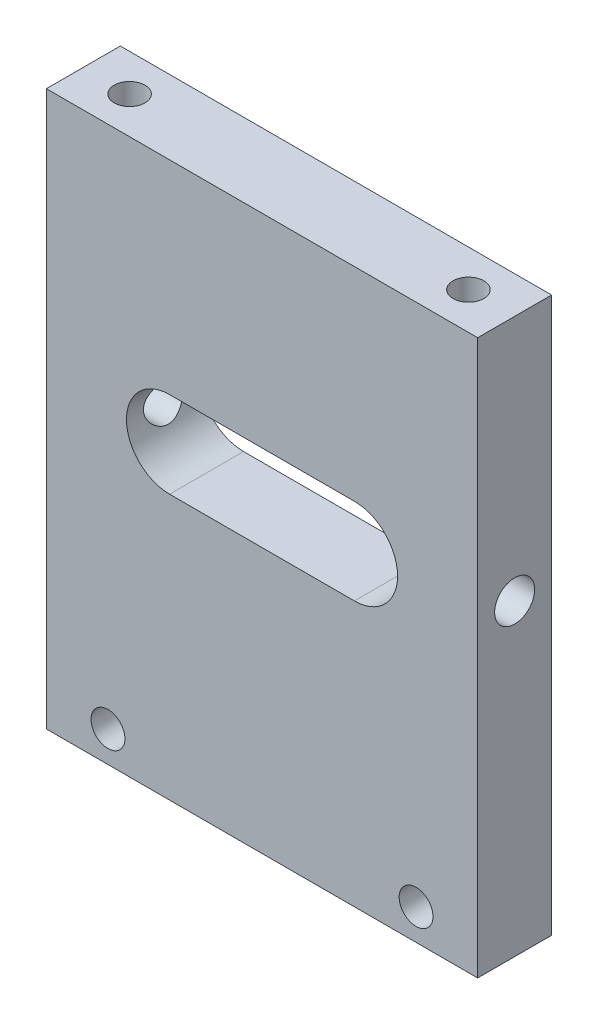
SolidWorks part; units mm, degrees
ref_plane "前视" through (0, 0, 0) normal (0, 0, 1) x (1, 0, 0)
ref_plane "上视" through (0, 0, 0) normal (0, 1, 0) x (1, 0, 0)
ref_plane "右视" through (0, 0, 0) normal (1, 0, 0) x (0, 0, -1)
sketch "草图1" plane through (0, 0, 0) normal (0, 0, 1) x (1, 0, 0)
  line L1 (0, 0) -> (70, 0)
  line L2 (0, 0) -> (0, -90)
  line L3 (0, -90) -> (70, -90)
  line L4 (70, 0) -> (70, -90)
  dimension "D1" = 70
  dimension "D2" = 90
extrude "凸台-拉伸1" add sketch "草图1" along normal blind 12
sketch "草图2" plane through (0, 0, 12) normal (0, 0, 1) x (1, 0, 0)
  line L0 (35, -40) -> (35, -90) construction
  line L1 (0, -90) -> (70, -90) construction
  line L2 (20, -40) -> (50, -40) construction
  line L3 (20, -33) -> (50, -33)
  line L4 (20, -47) -> (50, -47)
  arc A0 (20, -33) -> (20, -47) centre (20, -40) ccw
  arc A1 (50, -47) -> (50, -33) centre (50, -40) ccw
  point P6 (35, -40)
  dimension "D1" = 14
  dimension "D2" = 50
  dimension "D3" = 30
extrude "切除-拉伸1" cut sketch "草图2" against normal through all
sketch "草图4" plane through (70, 0, 0) normal (1, 0, 0) x (0, 0, -1)
  line L0 (-6, -40) -> (-6, -90) construction
  line L2 (-12, -90) -> (0, -90) construction
  circle A0 centre (-6, -40) radius 3.25
  dimension "D2" = 6.5
  dimension "D1" = 50
extrude "切除-拉伸2" cut sketch "草图4" against normal through all
cosmetic thread "装饰螺纹线1" parameters "D2"=8
cosmetic thread "装饰螺纹线2" parameters "D2"=8
hole_wizard "M6 螺纹孔1" positions "草图6" profile "草图5" tap size "M6" standard "GB"
sketch "草图6" plane through (0, 0, 0) normal (0, 1, 0) x (1, 0, 0)
  point P0 (62.5, -6)
  point P3 (7.5, -6)
sketch "草图5" plane through (62.5, 0, 6) normal (1, 0, 0) x (0, 0, 1)
  line L0 (0, 0) -> (0, 18.5022)
  line L1 (0, 18.5022) -> (2.5, 17)
  line L2 (2.5, 17) -> (2.5, 0)
  line L5 (2.5, 0) -> (0, 0)
  line L10 (0, 18.5022) -> (-2.5, 17) construction
  line L11 (0, -6.35) -> (0, 107.95) construction
  dimension "螺纹孔钻头直径" = 5
  dimension "螺纹孔钻头深度" = 17
  dimension "导头角度" = 118
cosmetic thread "孔螺蚊线1" parameters "D1"=12, "D2"=6
cosmetic thread "孔螺蚊线2" parameters "D1"=12, "D2"=6
sketch "草图11" plane through (0, 0, 12) normal (0, 0, 1) x (1, 0, 0)
  line L0 (10, -85) -> (60, -85) construction
  line L1 (35, -85) -> (35, -90) construction
  line L2 (0, -90) -> (70, -90) construction
  circle A0 centre (10, -85) radius 2.75
  circle A1 centre (60, -85) radius 2.75
  dimension "D3" = 5.5
  dimension "D1" = 50
  dimension "D2" = 5
extrude "切除-拉伸3" cut sketch "草图11" against normal through all
